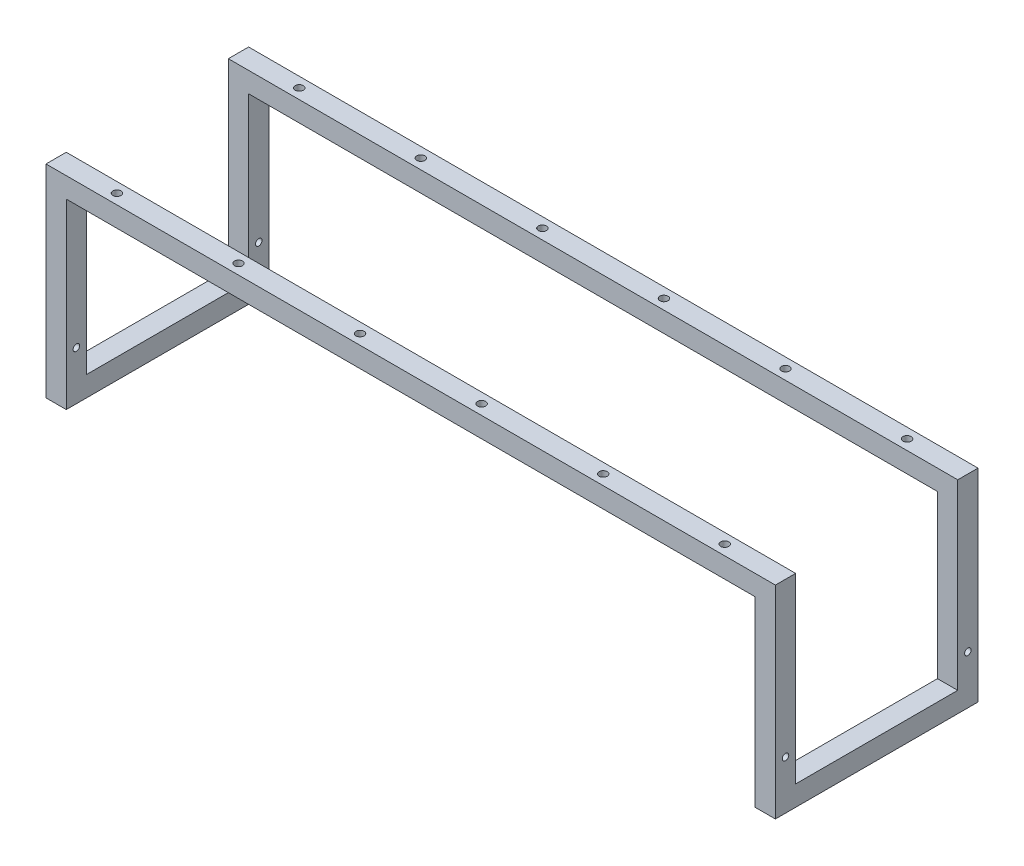
from build123d import *

# Parameters (mm, degrees)
SKETCH1_W               = 50
SKETCH1_H               = 50
BOSS_EXTRUDE1_DEPTH     = 500
SKETCH2_W               = 50
SKETCH2_H               = 50
BOSS_EXTRUDE2_DEPTH     = 450
SKETCH3_W               = 50
SKETCH3_H               = 50
BOSS_EXTRUDE3_DEPTH     = 1750
SKETCH4_W               = 50
SKETCH4_H               = 50
BOSS_EXTRUDE4_DEPTH     = 450
SKETCH5_W               = 50
SKETCH5_H               = 50
BOSS_EXTRUDE5_DEPTH     = 400
CUT_EXTRUDE1_REACH      = 1912.661
SKETCH6_R               = 10
LPATTERN1_COUNT         = 6
LPATTERN1_PITCH         = 300
SKETCH8_R               = 8
CUT_EXTRUDE2_DEPTH      = 1928.59565262
SKETCH9_W               = 15
SKETCH9_H               = 40
BOSS_EXTRUDE6_DEPTH     = 30
SKETCH12_W              = 15
SKETCH12_H              = 40
BOSS_EXTRUDE7_DEPTH     = 30
SKETCH13_W              = 15
SKETCH13_H              = 40
BOSS_EXTRUDE8_DEPTH     = 48
CUT_EXTRUDE3_DEPTH      = 1913.367642479
CUT_EXTRUDE3_DEPTH_BACK = 1913.367642479
SKETCH14_R              = 7.5
SKETCH15_R              = 7.5
SKETCH15_R_2            = 5.5
BOSS_EXTRUDE9_DEPTH     = 15


with BuildPart() as part:
    # Sketch1 → Boss-Extrude1 (new body)
    with BuildSketch(Plane.XY):
        Rectangle(SKETCH1_W, SKETCH1_H)
    extrude(amount=BOSS_EXTRUDE1_DEPTH)

    # Sketch2 → Boss-Extrude2 (add)
    with BuildSketch(Plane(origin=(0, 25, 0), x_dir=(1, 0, 0), z_dir=(0, 1, 0))):
        with Locations((0, -25)):
            Rectangle(SKETCH2_W, SKETCH2_H)
        with Locations((0, -475)):
            Rectangle(SKETCH2_W, SKETCH2_H)
    extrude(amount=BOSS_EXTRUDE2_DEPTH)

    # Sketch3 → Boss-Extrude3 (add)
    with BuildSketch(Plane(origin=(25, 0, 0), x_dir=(0, 0, -1), z_dir=(1, 0, 0))):
        with Locations((-475, 450)):
            Rectangle(SKETCH3_W, SKETCH3_H)
        with Locations((-25, 450)):
            Rectangle(SKETCH3_W, SKETCH3_H)
    extrude(amount=BOSS_EXTRUDE3_DEPTH)

    # Sketch4 → Boss-Extrude4 (add)
    with BuildSketch(Plane(origin=(0, 425, 0), x_dir=(-1, 0, 0), z_dir=(0, -1, 0))):
        with Locations((-1750, -475)):
            Rectangle(SKETCH4_W, SKETCH4_H)
        with Locations((-1750, -25)):
            Rectangle(SKETCH4_W, SKETCH4_H)
    extrude(amount=BOSS_EXTRUDE4_DEPTH)

    # Sketch5 → Boss-Extrude5 (add)
    with BuildSketch(Plane(origin=(0, 0, 450), x_dir=(-1, 0, 0), z_dir=(0, 0, -1))):
        with Locations((-1750, 0)):
            Rectangle(SKETCH5_W, SKETCH5_H)
    extrude(amount=BOSS_EXTRUDE5_DEPTH)

    # Sketch6 → Cut-Extrude1 (cut, up to next)
    with BuildSketch(Plane(origin=(0, 475, 0), x_dir=(1, 0, 0), z_dir=(0, 1, 0)), mode=Mode.PRIVATE) as cut_extrude1_sk1:
        with Locations(Location((125, -25, 0), (0, 0, 270))):
            Circle(SKETCH6_R)
    cut_extrude1_tool1 = extrude(cut_extrude1_sk1.sketch, amount=-CUT_EXTRUDE1_REACH, mode=Mode.PRIVATE) & part.part
    # Sketch6 → Cut-Extrude1 (cut, up to next)
    with BuildSketch(Plane(origin=(0, 475, 0), x_dir=(1, 0, 0), z_dir=(0, 1, 0)), mode=Mode.PRIVATE) as cut_extrude1_sk2:
        with Locations(Location((125, -475, 0), (0, 0, 270))):
            Circle(SKETCH6_R)
    cut_extrude1_tool2 = extrude(cut_extrude1_sk2.sketch, amount=-CUT_EXTRUDE1_REACH, mode=Mode.PRIVATE) & part.part
    cut_extrude1_1 = cut_extrude1_tool1.solids().sort_by_distance((125, 475, 25))[0]
    add(cut_extrude1_1, mode=Mode.SUBTRACT)
    cut_extrude1_2 = cut_extrude1_tool2.solids().sort_by_distance((125, 475, 475))[0]
    add(cut_extrude1_2, mode=Mode.SUBTRACT)
    cut_extrude1 = cut_extrude1_1 + cut_extrude1_2  # Cut-Extrude1 as one shape, for the pattern or mirror that repeats it

    # LPattern1: Cut-Extrude1 ×6
    with Locations(*[(i * LPATTERN1_PITCH, 0, 0) for i in range(1, LPATTERN1_COUNT)]):
        add(cut_extrude1, mode=Mode.SUBTRACT)

    # Sketch8 → Cut-Extrude2 (cut, through all)
    with BuildSketch(Plane.ZY.offset(25)):
        with Locations((475, 95)):
            Circle(SKETCH8_R)
        with Locations((25, 95)):
            Circle(SKETCH8_R)
    extrude(amount=-CUT_EXTRUDE2_DEPTH, mode=Mode.SUBTRACT)

    # Sketch9 → Boss-Extrude6 (add)
    with BuildSketch(Plane(origin=(0, 0, 450), x_dir=(-1, 0, 0), z_dir=(0, 0, -1))):
        with Locations((17.5, 95)):
            Rectangle(SKETCH9_W, SKETCH9_H)
    extrude(amount=BOSS_EXTRUDE6_DEPTH)

    # Sketch12 → Boss-Extrude7 (add)
    with BuildSketch(Plane(origin=(0, 0, 0), x_dir=(-1, 0, 0), z_dir=(0, 0, -1))):
        with Locations((17.5, 95)):
            Rectangle(SKETCH12_W, SKETCH12_H)
    extrude(amount=BOSS_EXTRUDE7_DEPTH)

    # Sketch13 → Boss-Extrude8 (add)
    with BuildSketch(Plane.ZY.offset(25)):
        with Locations((-22.5, 95)):
            Rectangle(SKETCH13_W, SKETCH13_H)
        with Locations((427.5, 95)):
            Rectangle(SKETCH13_W, SKETCH13_H)
    extrude(amount=BOSS_EXTRUDE8_DEPTH)

    # Sketch14 → Cut-Extrude3 (cut, two sides: drawn at the far end of the back side and taken through both)
    with BuildSketch(Plane(origin=(0, 0, -30), x_dir=(-1, 0, 0), z_dir=(0, 0, -1)).offset(-CUT_EXTRUDE3_DEPTH_BACK)):
        with Locations(Location((53, 95, 0), (0, 0, 90))):
            Circle(SKETCH14_R)
    extrude(amount=CUT_EXTRUDE3_DEPTH + CUT_EXTRUDE3_DEPTH_BACK, mode=Mode.SUBTRACT)

    # Sketch15 → Boss-Extrude9 (add)
    with BuildSketch(Plane(origin=(0, 0, -30), x_dir=(-1, 0, 0), z_dir=(0, 0, -1))):
        with Locations((53, 95)):
            Circle(SKETCH15_R)
        with Locations((53, 95)):
            Circle(SKETCH15_R_2, mode=Mode.SUBTRACT)
    extrude(amount=-BOSS_EXTRUDE9_DEPTH)


solid = part.part
